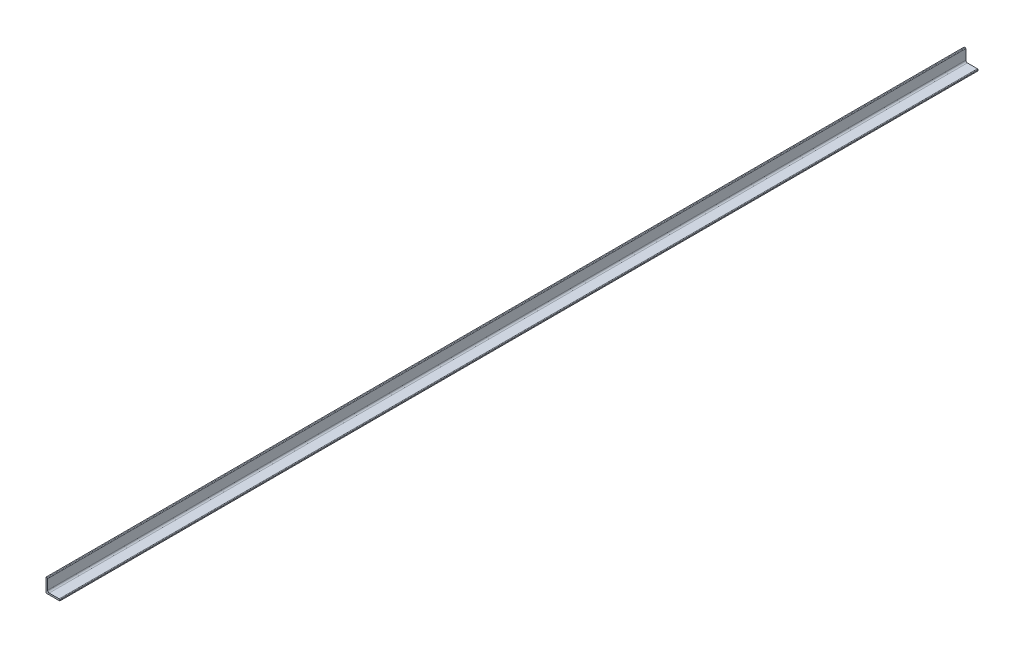
SolidWorks part; units mm, degrees
material "等边角钢70×8/Q235A"
ref_plane "Front Plane" through (0, 0, 0) normal (0, 0, 1) x (1, 0, 0)
ref_plane "Top Plane" through (0, 0, 0) normal (0, 1, 0) x (1, 0, 0)
ref_plane "Right Plane" through (0, 0, 0) normal (1, 0, 0) x (0, 0, -1)
sketch "Sketch1" plane through (0, 0, 0) normal (0, 0, 1) x (1, 0, 0)
  line L0 (0, 70) -> (0, 0)
  line L1 (0, 0) -> (70, 0)
  line L2 (70, 0) -> (70, 5)
  line L3 (67, 8) -> (16, 8)
  line L4 (8, 16) -> (8, 67)
  line L5 (5, 70) -> (0, 70)
  arc A0 (16, 8) -> (8, 16) centre (16, 16) cw
  arc A1 (70, 5) -> (67, 8) centre (67, 5) ccw
  arc A2 (8, 67) -> (5, 70) centre (5, 67) ccw
  dimension "D5" = 8
  dimension "D6" = 3
  dimension "D1" = 70
  dimension "D2" = 70
  dimension "D3" = 8
  dimension "D4" = 8
extrude "Boss-Extrude1" add sketch "Sketch1" along normal blind 4660
ref_plane "Plane1" through (0, 0, 0) normal (0.7071, 0.7071, 0) x (0, 0, -1)
